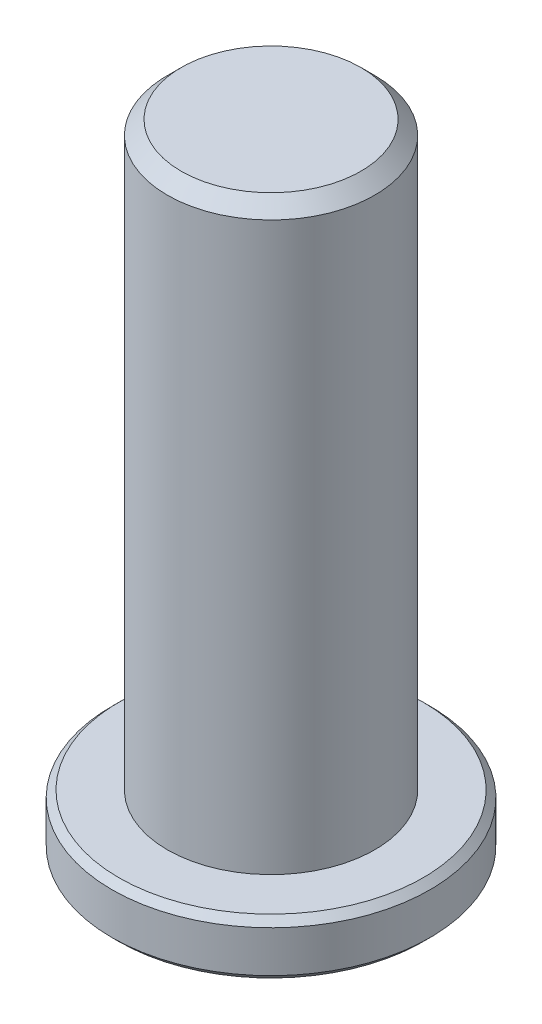
from build123d import *

# Parameters (mm, degrees)
SKETCH1_R           = 11.5
BOSS_EXTRUDE1_DEPTH = 4
SKETCH2_R           = 7.5
BOSS_EXTRUDE2_DEPTH = 42
CHAMFER1_SIZE       = 1
CHAMFER2_SIZE       = 0.5


with BuildPart() as part:
    # Sketch1 → Boss-Extrude1 (new body)
    with BuildSketch(Plane(origin=(0, 0, 0), x_dir=(1, 0, 0), z_dir=(0, 1, 0))):
        with Locations(Location((0, 0, 0), (0, 0, 270))):
            Circle(SKETCH1_R)
    extrude(amount=BOSS_EXTRUDE1_DEPTH)

    # Sketch2 → Boss-Extrude2 (add)
    with BuildSketch(Plane(origin=(0, 4, 0), x_dir=(1, 0, 0), z_dir=(0, 1, 0))):
        with Locations(Location((0, 0, 0), (0, 0, 90))):
            Circle(SKETCH2_R)
    extrude(amount=BOSS_EXTRUDE2_DEPTH)

    # Chamfer1
    chamfer1_edges = [part.edges().sort_by_distance(p)[0] for p in [
        (0, 46, 7.5),
    ]]
    chamfer(chamfer1_edges, length=CHAMFER1_SIZE)

    # Chamfer2
    chamfer2_edges = [part.edges().sort_by_distance(p)[0] for p in [
        (0, 0, -11.5),
        (0, 4, -11.5),
    ]]
    chamfer(chamfer2_edges, length=CHAMFER2_SIZE)


solid = part.part
